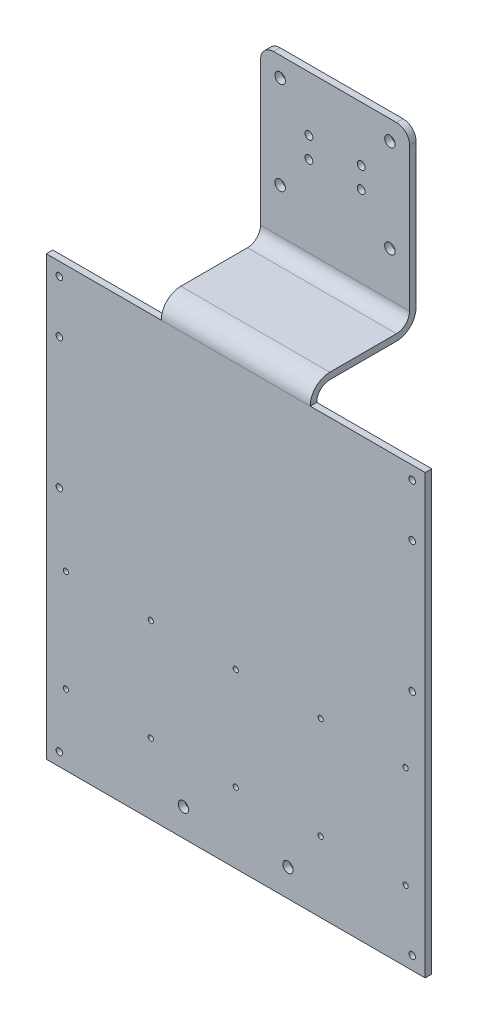
SolidWorks part; units mm, degrees
ref_plane "Front Plane" through (0, 0, 0) normal (0, 0, 1) x (1, 0, 0)
ref_plane "Top Plane" through (0, 0, 0) normal (0, 1, 0) x (1, 0, 0)
ref_plane "Right Plane" through (0, 0, 0) normal (1, 0, 0) x (0, 0, -1)
sketch "Sketch1" plane through (0, 0, 0) normal (0, 0, 1) x (1, 0, 0)
  line L1 (-145, -175) -> (145, -175)
  line L2 (-145, -175) -> (-145, 175)
  line L3 (-145, 175) -> (145, 175)
  line L4 (145, -175) -> (145, 175)
  line L5 (-145, -175) -> (145, 175) construction
  line L6 (-145, 175) -> (145, -175) construction
  point P0 (0, 0)
  dimension "D1" = 290
  dimension "D2" = 350
extrude "Boss-Extrude1" add sketch "Sketch1" along normal blind 5
sketch "Sketch2" plane through (0, 0, 5) normal (0, 0, 1) x (1, 0, 0)
  line L0 (145, 175) -> (-145, 175) construction
  line L1 (-57, 175) -> (57, 175)
  line L2 (-57, 175) -> (-57, 170)
  line L3 (-57, 170) -> (57, 170)
  line L4 (57, 175) -> (57, 170)
  line L5 (-145, 175) -> (-145, -175) construction
  dimension "D1" = 5
  dimension "D2" = 114
  dimension "D3" = 88
extrude "Boss-Extrude2" add sketch "Sketch2" against normal blind 81
sketch "Sketch3" plane through (0, 170, 0) normal (0, -1, 0) x (-1, 0, 0)
  line L0 (57, 76) -> (57, 0) construction
  line L1 (-57, 76) -> (57, 76)
  line L2 (-57, 76) -> (-57, 71)
  line L3 (-57, 71) -> (57, 71)
  line L4 (57, 76) -> (57, 71)
  dimension "D1" = 5
extrude "Boss-Extrude3" add sketch "Sketch3" against normal blind 135
fillet "Fillet1" radius 10 2 edges at (0, 175, -71) (0, 170, 0)
sketch "Sketch4" plane through (0, 0, 0) normal (0, 0, -1) x (-1, 0, 0)
  line L1 (57, 160) -> (145, 160)
  line L2 (57, 160) -> (57, 175)
  line L3 (57, 175) -> (145, 175)
  line L4 (145, 160) -> (145, 175)
  line L5 (-57, 160) -> (-145, 160)
  line L6 (-57, 160) -> (-57, 175)
  line L7 (-57, 175) -> (-145, 175)
  line L8 (-145, 160) -> (-145, 175)
extrude "Cut-Extrude1" cut sketch "Sketch4" against normal blind 120
fillet "Fillet2" radius 15 2 edges at (0, 175, 5) (0, 170, -76)
fillet "Fillet3" radius 10 2 edges at (-57, 305, -73.5) (57, 305, -73.5)
sketch "Sketch5" plane through (0, 0, -76) normal (0, 0, -1) x (-1, 0, 0)
  line L0 (57, 295) -> (57, 185) construction
  line L2 (47, 305) -> (-47, 305) construction
  line L3 (-57, 185) -> (-57, 295) construction
  circle A0 centre (42, 290) radius 4
  circle A1 centre (-42, 290) radius 4
  circle A2 centre (42, 219) radius 4
  circle A3 centre (-42, 219) radius 4
  dimension "D1" = 8
  dimension "D2" = 8
  dimension "D3" = 8
  dimension "D4" = 8
  dimension "D5" = 71
  dimension "D6" = 84
  dimension "D7" = 15
  dimension "D8" = 15
  dimension "D9" = 15
  dimension "D10" = 71
  dimension "D11" = 84
  dimension "D12" = 15
extrude "Cut-Extrude2" cut sketch "Sketch5" against normal blind 120
sketch "Sketch7" plane through (0, 0, 0) normal (0, 0, -1) x (-1, 0, 0)
  circle A0 centre (-130, -121) radius 2
  circle A1 centre (-65, -121) radius 2
  circle A2 centre (0, -121) radius 2
  circle A3 centre (65, -121) radius 2
  circle A4 centre (130, -121) radius 2
  circle A5 centre (130, -43) radius 2
  circle A6 centre (65, -43) radius 2
  circle A7 centre (0, -43) radius 2
  circle A8 centre (-65, -43) radius 2
  circle A9 centre (-130, -43) radius 2
extrude "Cut-Extrude3" cut sketch "Sketch7" against normal blind 10
sketch "Sketch8" plane through (0, 0, -76) normal (0, 0, -1) x (-1, 0, 0)
  circle A0 centre (-20, 247) radius 3
  circle A1 centre (-20, 263) radius 3
  circle A2 centre (20, 263) radius 3
  circle A3 centre (20, 247) radius 3
extrude "Cut-Extrude4" cut sketch "Sketch8" against normal blind 10
sketch "Sketch9" plane through (0, 0, 0) normal (0, 0, -1) x (-1, 0, 0)
  circle A0 centre (40, -154) radius 4
  circle A1 centre (-40, -154) radius 4
extrude "Cut-Extrude5" cut sketch "Sketch9" against normal blind 10
sketch "Sketch10" plane through (0, 0, 0) normal (0, 0, -1) x (-1, 0, 0)
  circle A0 centre (-135, -165) radius 2.5
  circle A1 centre (135, -165) radius 2.5
  circle A2 centre (135, 150) radius 2.5
  circle A3 centre (-135, 150) radius 2.5
extrude "Cut-Extrude6" cut sketch "Sketch10" against normal blind 10
sketch "Sketch11" plane through (0, 0, 0) normal (0, 0, -1) x (-1, 0, 0)
  circle A0 centre (135, 110) radius 2.5
  circle A1 centre (135, 10) radius 2.5
  circle A2 centre (-135, 110) radius 2.5
  circle A3 centre (-135, 10) radius 2.5
extrude "Cut-Extrude7" cut sketch "Sketch11" against normal blind 10
